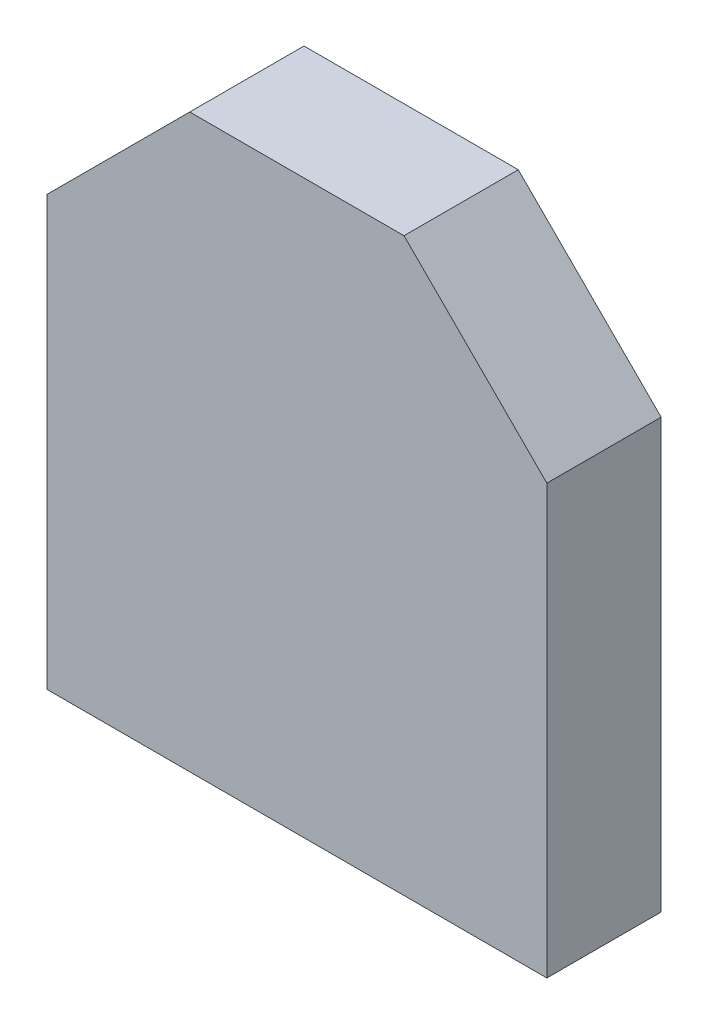
SolidWorks part; units mm, degrees
ref_plane "Front Plane" through (0, 0, 0) normal (0, 0, 1) x (1, 0, 0)
ref_plane "Top Plane" through (0, 0, 0) normal (0, 1, 0) x (1, 0, 0)
ref_plane "Right Plane" through (0, 0, 0) normal (1, 0, 0) x (0, 0, -1)
sketch "Sketch1" plane through (0, 0, 0) normal (0, 0, 1) x (1, 0, 0)
  line L0 (0, 30) -> (10, 40)
  line L1 (0, 0) -> (35, 0)
  line L2 (0, 0) -> (0, 30)
  line L3 (10, 40) -> (25, 40)
  line L4 (35, 0) -> (35, 30)
  line L5 (25, 40) -> (35, 30)
  point P1 (35, 40)
  point P2 (0, 40)
  dimension "D1" = 35
  dimension "D2" = 40
extrude "Boss-Extrude1" add sketch "Sketch1" along normal blind 8
